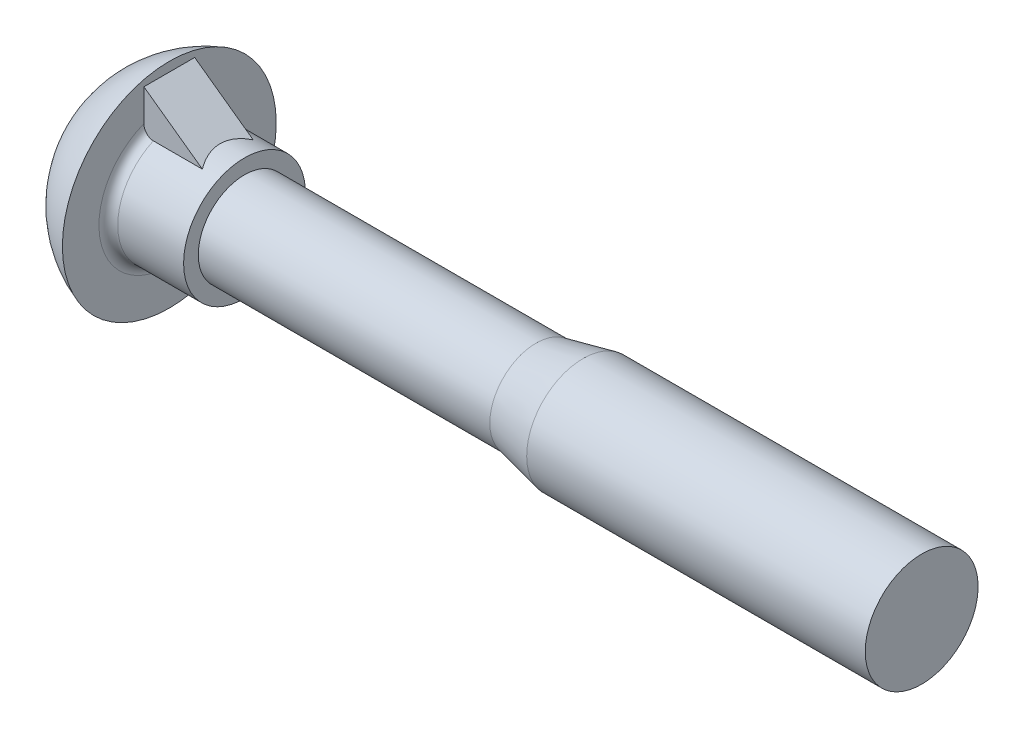
SolidWorks part; units mm, degrees
ref_plane "Front" through (0, 0, 0) normal (0, 0, 1) x (1, 0, 0)
ref_plane "Top" through (0, 0, 0) normal (0, 1, 0) x (1, 0, 0)
ref_plane "Right" through (0, 0, 0) normal (1, 0, 0) x (0, 0, -1)
other "Configuration Table"
sketch "Sketch1" plane through (0, 0, 0) normal (0, 0, 1) x (1, 0, 0)
  line L0 (-31.4843, 0) -> (43.5502, 0) construction
  line L1 (44.08, 0) -> (44.08, 3)
  line L2 (44.08, 3) -> (8.08, 3)
  line L3 (8.08, 3) -> (8.08, 3.24)
  line L4 (8.08, 3.24) -> (4.58, 3.24)
  line L5 (4.08, 3.74) -> (4.08, 5.6845)
  line L6 (44.08, 0) -> (0, 0)
  arc A0 (4.08, 5.6845) -> (0, 0) centre (6, 0) ccw
  arc A1 (4.58, 3.24) -> (4.08, 3.74) centre (4.58, 3.74) cw
  point P13 (4.08, 3.24)
revolve "Base" add sketch "Sketch1" angle 360 about L0
cosmetic thread "ThreadCosmetic1" [suppressed] parameters "D2"=4.917
sketch "Sketch2" plane through (0, 0, 0) normal (0, 0, 1) x (1, 0, 0)
  line L1 (6.78, 3.24) -> (4.08, 5.1845)
  line L2 (8.08, 3.24) -> (4.58, 3.24) construction
  line L3 (4.08, -5.6845) -> (4.08, 5.6845) construction
  line L4 (-31.4843, 0) -> (43.5502, 0) construction
rib "Nib" sketch "Sketch2" sketch "Sketch2" thickness 2.7 extrusion direction parallel to sketch draft on no parameters "Sn"=2.7
sketch "Sketch3" plane through (0, 0, 0) normal (0, 0, 1) x (1, 0, 0)
  line L0 (26.08, 3) -> (23.58, 2.4585)
  line L1 (0, 0) -> (55.457, 0) construction
  line L2 (23.58, 2.4585) -> (8.08, 2.4585)
  line L3 (44.08, -3) -> (44.08, 3) construction
  line L4 (8.08, 2.4585) -> (8.08, 3)
  line L5 (8.08, 3) -> (26.08, 3)
  line L6 (-29.8163, 0) -> (1.1759, 0) construction
revolve "Cut-Revolve1" cut sketch "Sketch3" angle 360 about L6
sketch "Sketch4" plane through (0, 0, 0) normal (0, 0, 1) x (1, 0, 0)
  line L0 (43.8092, 3.2) -> (44.3507, 3.2)
  line L1 (44.3507, 3.2) -> (44.3507, 3)
  line L2 (44.3507, 3) -> (44.08, 2.531)
  line L3 (44.08, -3) -> (44.08, 3) construction
  line L5 (43.8092, 3) -> (44.08, 2.531)
  line L6 (43.8092, 3.2) -> (43.8092, 3)
  line L8 (44.08, 0) -> (39.6447, 0) construction
  line L9 (43.8092, 3) -> (44.3507, 3) construction
  line L10 (44.08, 3) -> (44.08, 2.531) construction
  point P10 (44.08, 3.2)
revolve "Cut-Revolve10" [suppressed] cut sketch "Sketch4" angle 360 about L8
pattern_linear "LPattern10" [suppressed] count 55 spacing 0.6498 along (1, 0, 0)
equation "\"D2@Sketch2\" = sqr ( \"r@Sketch1\" * \"r@Sketch1\" -  ( \"r@Sketch1\" - \"k@Sketch1\" )  *  ( \"r@Sketch1\" - \"k@Sketch1\" )  ) -0.5"
equation "\"D2@Sketch4\" =  ( \"d@Sketch1\" - \"D2@ThreadCosmetic1\" )  / 2"
equation "\"D3@LPattern10\" = 1.2 * \"D2@Sketch4\" "
equation "\"D1@LPattern10\" =  ( \"l@Sketch1\" - \"h@Sketch1\" )  /  \"D3@LPattern10\""
equation "\"D1@Sketch3\" = \"D2@ThreadCosmetic1\""
equation "\"D3@Sketch4\" = \"d@Sketch1\""
